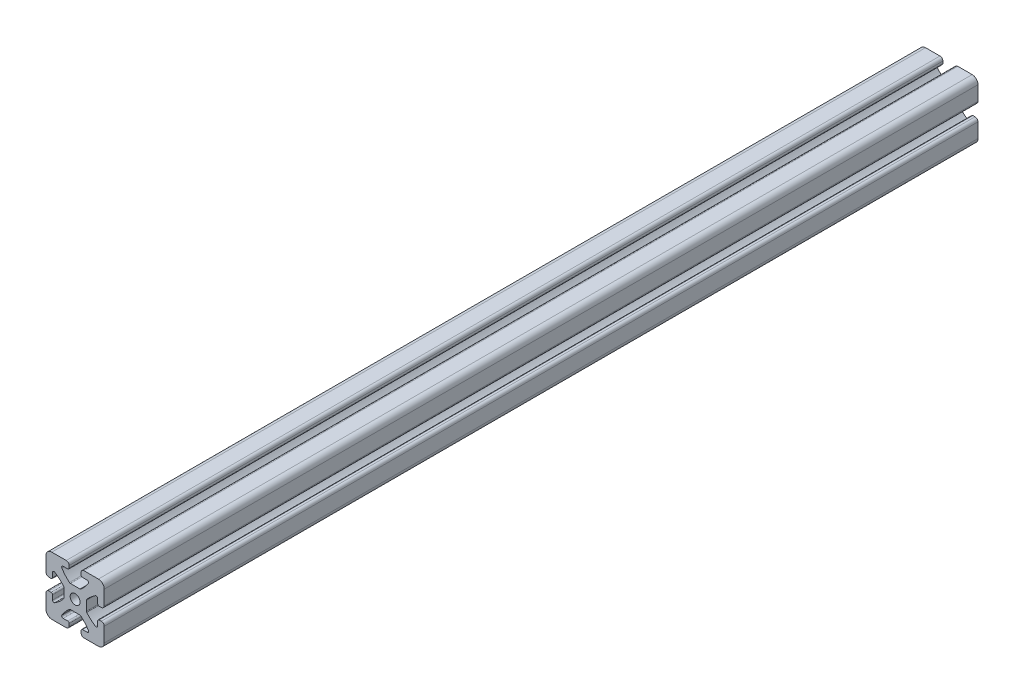
SolidWorks part; units mm, degrees
ref_plane "Front Plane" through (0, 0, 0) normal (0, 0, 1) x (1, 0, 0)
ref_plane "Top Plane" through (0, 0, 0) normal (0, 1, 0) x (1, 0, 0)
ref_plane "Right Plane" through (0, 0, 0) normal (1, 0, 0) x (0, 0, -1)
sketch "Sketch1" plane through (0, 0, 0) normal (0, 0, 1) x (1, 0, 0)
  line L0 (-75.7088, -20.1458) -> (-72.5526, -20.1458)
  line L1 (-70.701, -12.3958) -> (-67.4526, -12.3958)
  line L2 (-96.3499, -4.6458) -> (-39.5519, -4.6458) construction
  line L3 (-87.4526, 11.3542) -> (-87.4526, 1.3542)
  line L4 (-83.4526, -24.6458) -> (-73.5526, -24.6458)
  line L5 (-87.4526, -10.6458) -> (-87.4526, -20.6458)
  line L6 (-83.4526, 15.3542) -> (-73.4526, 15.3542)
  line L7 (-47.4526, -10.6458) -> (-47.4526, -20.6458)
  line L8 (-51.4526, -24.6458) -> (-61.4526, -24.6458)
  line L9 (-59.1964, -20.1458) -> (-62.4526, -20.1458)
  line L10 (-51.4526, 15.3542) -> (-61.4526, 15.3542)
  line L11 (-47.4526, 11.3542) -> (-47.4526, 1.3542)
  line L12 (-64.2043, -12.3958) -> (-67.4526, -12.3958)
  line L13 (-71.5526, -21.1458) -> (-71.5526, -22.6458)
  line L14 (-63.3526, -21.1458) -> (-63.3526, -22.6458)
  line L15 (-50.9526, -8.7458) -> (-49.4526, -8.7458)
  line L16 (-51.9526, -12.902) -> (-51.9526, -9.7458)
  line L17 (-59.7026, -7.8942) -> (-59.7026, -4.6458)
  line L18 (-50.9526, -0.5458) -> (-49.4526, -0.5458)
  line L19 (-51.9526, 3.6104) -> (-51.9526, 0.3542)
  line L20 (-59.7026, -1.3975) -> (-59.7026, -4.6458)
  line L21 (-63.3526, 11.8542) -> (-63.3526, 13.3542)
  line L22 (-59.1964, 10.8542) -> (-62.3526, 10.8542)
  line L23 (-63.8526, 3.1042) -> (-67.4526, 3.1042)
  line L24 (-71.5526, 11.8542) -> (-71.5526, 13.3542)
  line L25 (-75.7088, 10.8542) -> (-72.4526, 10.8542)
  line L26 (-71.0526, 3.1042) -> (-67.4526, 3.1042)
  line L27 (-83.9526, -0.5458) -> (-85.4526, -0.5458)
  line L28 (-82.9526, 3.6104) -> (-82.9526, 0.4542)
  line L29 (-75.2026, -1.3975) -> (-75.2026, -4.6458)
  line L30 (-83.9526, -8.7458) -> (-85.4526, -8.7458)
  line L31 (-82.9526, -12.902) -> (-82.9526, -9.6458)
  line L32 (-75.2026, -7.8942) -> (-75.2026, -4.6458)
  line L33 (-67.4526, 16.4313) -> (-67.4526, -26.9314) construction
  arc A0 (-71.3325, -12.6205) -> (-76.5532, -18.6101) centre (-55.648, -31.5616) ccw
  arc A1 (-76.5532, -18.6101) -> (-75.7088, -20.1458) centre (-75.7088, -19.1458) ccw
  arc A2 (-70.701, -12.3958) -> (-71.3325, -12.6205) centre (-70.701, -13.3958) ccw
  arc A3 (-83.4526, 15.3542) -> (-87.4526, 11.3542) centre (-83.4526, 11.3542) ccw
  arc A4 (-87.4526, -20.6458) -> (-83.4526, -24.6458) centre (-83.4526, -20.6458) ccw
  arc A6 (-63.5727, -12.6205) -> (-64.2043, -12.3958) centre (-64.2043, -13.3958) ccw
  arc A7 (-58.352, -18.6101) -> (-63.5727, -12.6205) centre (-79.2572, -31.5616) ccw
  arc A8 (-59.1964, -20.1458) -> (-58.352, -18.6101) centre (-59.1964, -19.1458) ccw
  arc A9 (-51.4526, -24.6458) -> (-47.4526, -20.6458) centre (-51.4526, -20.6458) ccw
  arc A10 (-47.4526, 11.3542) -> (-51.4526, 15.3542) centre (-51.4526, 11.3542) ccw
  circle A11 centre (-67.4526, -4.6458) radius 3.4
  arc A12 (-71.5526, -21.1458) -> (-72.5526, -20.1458) centre (-72.5526, -21.1458) ccw
  arc A13 (-73.5526, -24.6458) -> (-71.5526, -22.6458) centre (-73.5526, -22.6458) ccw
  arc A14 (-62.3526, -20.1458) -> (-63.3526, -21.1458) centre (-62.3526, -21.1458) ccw
  arc A15 (-63.3526, -22.6458) -> (-61.3526, -24.6458) centre (-61.3526, -22.6458) ccw
  arc A16 (-59.7026, -7.8942) -> (-59.478, -8.5257) centre (-58.7026, -7.8942) ccw
  arc A17 (-59.478, -8.5257) -> (-53.4884, -13.7464) centre (-40.5368, 7.1588) ccw
  arc A18 (-53.4884, -13.7464) -> (-51.9526, -12.902) centre (-52.9526, -12.902) ccw
  arc A19 (-50.9526, -8.7458) -> (-51.9526, -9.7458) centre (-50.9526, -9.7458) ccw
  arc A20 (-47.4526, -10.7458) -> (-49.4526, -8.7458) centre (-49.4526, -10.7458) ccw
  arc A21 (-59.478, -0.7659) -> (-59.7026, -1.3975) centre (-58.7026, -1.3975) ccw
  arc A22 (-53.4884, 4.4548) -> (-59.478, -0.7659) centre (-40.5368, -16.4504) ccw
  arc A23 (-51.9526, 0.4542) -> (-50.9526, -0.5458) centre (-50.9526, 0.4542) ccw
  arc A24 (-49.4526, -0.5458) -> (-47.4526, 1.4542) centre (-49.4526, 1.4542) ccw
  arc A25 (-51.9526, 3.6104) -> (-53.4884, 4.4548) centre (-52.9526, 3.6104) ccw
  arc A26 (-64.2043, 3.1042) -> (-63.5727, 3.3289) centre (-64.2043, 4.1042) ccw
  arc A27 (-63.5727, 3.3289) -> (-58.352, 9.3184) centre (-79.2572, 22.27) ccw
  arc A28 (-58.352, 9.3184) -> (-59.1964, 10.8542) centre (-59.1964, 9.8542) ccw
  arc A29 (-63.3526, 11.8542) -> (-62.3526, 10.8542) centre (-62.3526, 11.8542) ccw
  arc A30 (-61.3526, 15.3542) -> (-63.3526, 13.3542) centre (-61.3526, 13.3542) ccw
  arc A31 (-71.3325, 3.3289) -> (-70.701, 3.1042) centre (-70.701, 4.1042) ccw
  arc A32 (-76.5532, 9.3184) -> (-71.3325, 3.3289) centre (-55.648, 22.27) ccw
  arc A33 (-72.5526, 10.8542) -> (-71.5526, 11.8542) centre (-72.5526, 11.8542) ccw
  arc A34 (-71.5526, 13.3542) -> (-73.5526, 15.3542) centre (-73.5526, 13.3542) ccw
  arc A35 (-75.7088, 10.8542) -> (-76.5532, 9.3184) centre (-75.7088, 9.8542) ccw
  arc A36 (-75.2026, -1.3975) -> (-75.4273, -0.7659) centre (-76.2026, -1.3975) ccw
  arc A37 (-75.4273, -0.7659) -> (-81.4169, 4.4548) centre (-94.3684, -16.4504) ccw
  arc A38 (-81.4169, 4.4548) -> (-82.9526, 3.6104) centre (-81.9526, 3.6104) ccw
  arc A39 (-83.9526, -0.5458) -> (-82.9526, 0.4542) centre (-83.9526, 0.4542) ccw
  arc A40 (-87.4526, 1.4542) -> (-85.4526, -0.5458) centre (-85.4526, 1.4542) ccw
  arc A41 (-75.4273, -8.5257) -> (-75.2026, -7.8942) centre (-76.2026, -7.8942) ccw
  arc A42 (-81.4169, -13.7464) -> (-75.4273, -8.5257) centre (-94.3684, 7.1588) ccw
  arc A43 (-82.9526, -9.7458) -> (-83.9526, -8.7458) centre (-83.9526, -9.7458) ccw
  arc A44 (-85.4526, -8.7458) -> (-87.4526, -10.7458) centre (-85.4526, -10.7458) ccw
  arc A45 (-82.9526, -12.902) -> (-81.4169, -13.7464) centre (-81.9526, -12.902) ccw
extrude "Boss-Extrude1" add sketch "Sketch1" along normal blind 600 contours A45 L31 A43 L30 A44 L5 A4 L4 A13 L13 A12 L0 A1 A0 A2 L1 L12 A6 A7 A8 L9 A14 L14 A15 L8 A9 L7 A20 L15 A19 L16 A18 A17 A16 L17 L20 A21 A22 A25 L19 A23 L18 A24 L11 A10 L10 A30 L21 A29 L22 A28
